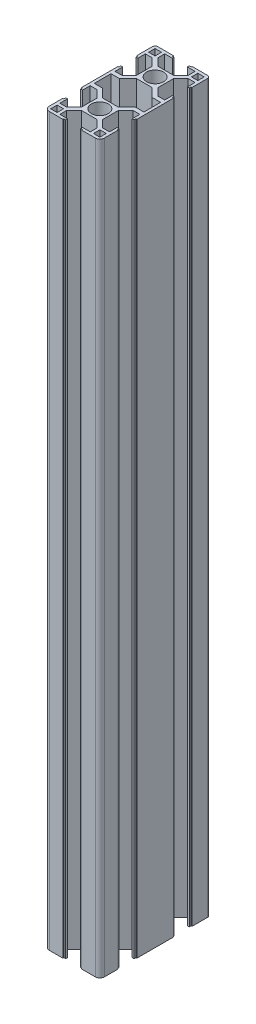
from build123d import *

# Parameters (mm, degrees)
SKETCH1_R                                = 4.6
SKETCH1_W                                = 3.5
SKETCH1_H                                = 3.5
ALUMINUM_PROFILE_30_X_60L_X_R2_5_1_DEPTH = 395


with BuildPart() as part:
    # Sketch1 → Aluminum profile 30 X 60L X R2.5(1) (new body)
    with BuildSketch(Plane(origin=(0, 0, 0), x_dir=(-1, 0, 0), z_dir=(0, 1, 0))):
        with BuildLine():
            Line((-5.1, 15), (-5.1, 14.5))
            Line((-5.1, 14.5), (-4.1, 14.5))
            Line((-4.1, 14.5), (-4.1, 13.5))
            Line((-4.1, 13.5), (-8.25, 13.5))
            Line((-8.25, 13.5), (-8.25, 9.8))
            Line((-8.25, 9.8), (-4.25, 5.8))
            Line((-4.25, 5.8), (4.25, 5.8))
            Line((4.25, 5.8), (8.25, 9.8))
            Line((8.25, 9.8), (8.25, 13.5))
            Line((8.25, 13.5), (4.1, 13.5))
            Line((4.1, 13.5), (4.1, 14.5))
            Line((4.1, 14.5), (5.1, 14.5))
            Line((5.1, 14.5), (5.1, 15))
            Line((5.1, 15), (12.5, 15))
            ThreePointArc((12.5, 15), (14.267766953, 14.267766953), (15, 12.5))
            Line((15, 12.5), (15, 5.1))
            Line((15, 5.1), (14.5, 5.1))
            Line((14.5, 5.1), (14.5, 4.1))
            Line((14.5, 4.1), (13.5, 4.1))
            Line((13.5, 4.1), (13.5, 8.25))
            Line((13.5, 8.25), (9.8, 8.25))
            Line((9.8, 8.25), (5.8, 4.25))
            Line((5.8, 4.25), (5.8, -4.25))
            Line((5.8, -4.25), (9.8, -8.25))
            Line((9.8, -8.25), (13.5, -8.25))
            Line((13.5, -8.25), (13.5, -4.1))
            Line((13.5, -4.1), (14.5, -4.1))
            Line((14.5, -4.1), (14.5, -5.1))
            Line((14.5, -5.1), (15, -5.1))
            Line((15, -5.1), (15, -24.9))
            Line((15, -24.9), (14.5, -24.9))
            Line((14.5, -24.9), (14.5, -25.9))
            Line((14.5, -25.9), (13.5, -25.9))
            Line((13.5, -25.9), (13.5, -21.75))
            Line((13.5, -21.75), (9.8, -21.75))
            Line((9.8, -21.75), (5.8, -25.75))
            Line((5.8, -25.75), (5.8, -34.25))
            Line((5.8, -34.25), (9.8, -38.25))
            Line((9.8, -38.25), (13.5, -38.25))
            Line((13.5, -38.25), (13.5, -34.1))
            Line((13.5, -34.1), (14.5, -34.1))
            Line((14.5, -34.1), (14.5, -35.1))
            Line((14.5, -35.1), (15, -35.1))
            Line((15, -35.1), (15, -43.5))
            ThreePointArc((15, -43.5), (14.560660172, -44.560660172), (13.5, -45))
            Line((13.5, -45), (5.1, -45))
            Line((5.1, -45), (5.1, -44.5))
            Line((5.1, -44.5), (4.1, -44.5))
            Line((4.1, -44.5), (4.1, -43.5))
            Line((4.1, -43.5), (8.25, -43.5))
            Line((8.25, -43.5), (8.25, -39.8))
            Line((8.25, -39.8), (4.25, -35.8))
            Line((4.25, -35.8), (-4.25, -35.8))
            Line((-4.25, -35.8), (-8.25, -39.8))
            Line((-8.25, -39.8), (-8.25, -43.5))
            Line((-8.25, -43.5), (-4.1, -43.5))
            Line((-4.1, -43.5), (-4.1, -44.5))
            Line((-4.1, -44.5), (-5.1, -44.5))
            Line((-5.1, -44.5), (-5.1, -45))
            Line((-5.1, -45), (-13.5, -45))
            ThreePointArc((-13.5, -45), (-14.560660172, -44.560660172), (-15, -43.5))
            Line((-15, -43.5), (-15, -35.1))
            Line((-15, -35.1), (-14.5, -35.1))
            Line((-14.5, -35.1), (-14.5, -34.1))
            Line((-14.5, -34.1), (-13.5, -34.1))
            Line((-13.5, -34.1), (-13.5, -38.25))
            Line((-13.5, -38.25), (-9.8, -38.25))
            Line((-9.8, -38.25), (-5.8, -34.25))
            Line((-5.8, -34.25), (-5.8, -25.75))
            Line((-5.8, -25.75), (-9.8, -21.75))
            Line((-9.8, -21.75), (-13.5, -21.75))
            Line((-13.5, -21.75), (-13.5, -25.9))
            Line((-13.5, -25.9), (-14.5, -25.9))
            Line((-14.5, -25.9), (-14.5, -24.9))
            Line((-14.5, -24.9), (-15, -24.9))
            Line((-15, -24.9), (-15, -5.1))
            Line((-15, -5.1), (-14.5, -5.1))
            Line((-14.5, -5.1), (-14.5, -4.1))
            Line((-14.5, -4.1), (-13.5, -4.1))
            Line((-13.5, -4.1), (-13.5, -8.25))
            Line((-13.5, -8.25), (-9.8, -8.25))
            Line((-9.8, -8.25), (-5.8, -4.25))
            Line((-5.8, -4.25), (-5.8, 4.25))
            Line((-5.8, 4.25), (-9.8, 8.25))
            Line((-9.8, 8.25), (-13.5, 8.25))
            Line((-13.5, 8.25), (-13.5, 4.1))
            Line((-13.5, 4.1), (-14.5, 4.1))
            Line((-14.5, 4.1), (-14.5, 5.1))
            Line((-14.5, 5.1), (-15, 5.1))
            Line((-15, 5.1), (-15, 12.5))
            ThreePointArc((-15, 12.5), (-14.267766953, 14.267766953), (-12.5, 15))
            Line((-12.5, 15), (-5.1, 15))
        make_face()
        Circle(SKETCH1_R, mode=Mode.SUBTRACT)
        with Locations((0, -30)):
            Circle(SKETCH1_R, mode=Mode.SUBTRACT)
        Polygon((8.9, -10.45), (4.25, -5.8), (-4.25, -5.8), (-8.9, -10.45), (-13.5, -10.45), (-13.5, -19.55), (-8.9, -19.55), (-4.25, -24.2), (4.25, -24.2), (8.9, -19.55), (13.5, -19.55), (13.5, -10.45), align=None, mode=Mode.SUBTRACT)
        with Locations((-11.625, 11.625)):
            Rectangle(SKETCH1_W, SKETCH1_H, mode=Mode.SUBTRACT)
        with Locations((11.625, 11.625)):
            Rectangle(SKETCH1_W, SKETCH1_H, mode=Mode.SUBTRACT)
        with Locations((-11.625, -41.625)):
            Rectangle(SKETCH1_W, SKETCH1_H, mode=Mode.SUBTRACT)
        with Locations((11.625, -41.625)):
            Rectangle(SKETCH1_W, SKETCH1_H, mode=Mode.SUBTRACT)
    extrude(amount=ALUMINUM_PROFILE_30_X_60L_X_R2_5_1_DEPTH)


solid = part.part
